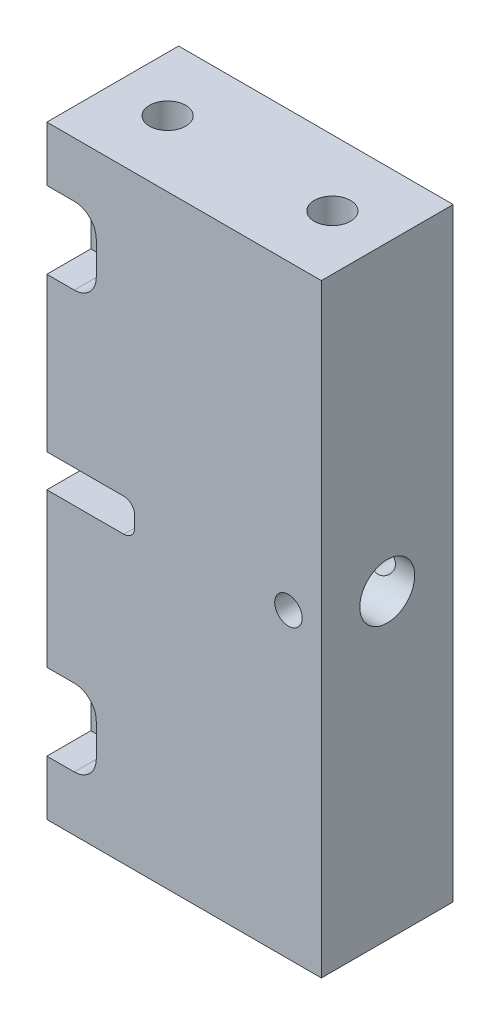
SolidWorks part; units mm, degrees
material "6061铝"
ref_plane "前视基准面" through (0, 0, 0) normal (0, 0, 1) x (1, 0, 0)
ref_plane "上视基准面" through (0, 0, 0) normal (0, 1, 0) x (1, 0, 0)
ref_plane "右视基准面" through (0, 0, 0) normal (1, 0, 0) x (0, 0, -1)
sketch "草图1" plane through (0, 0, 0) normal (1, 0, 0) x (0, 0, -1)
  line L1 (-6, 27.5) -> (6, 27.5)
  line L2 (-6, 27.5) -> (-6, -27.5)
  line L3 (-6, -27.5) -> (6, -27.5)
  line L4 (6, 27.5) -> (6, -27.5)
  line L5 (-6, 27.5) -> (6, -27.5) construction
  line L6 (-6, -27.5) -> (6, 27.5) construction
  point P0 (0, 0)
  dimension "D1" = 12
  dimension "D2" = 55
extrude "凸台-拉伸1" add sketch "草图1" along normal blind 25
sketch "草图2" plane through (25, 0, 0) normal (1, 0, 0) x (0, 0, -1)
  circle A0 centre (0, 0) radius 1.1
  dimension "D1" = 2.2
extrude "切除-拉伸1" cut sketch "草图2" against normal blind 25
sketch "草图3" plane through (25, 0, 0) normal (1, 0, 0) x (0, 0, -1)
  circle A0 centre (0, 0) radius 2.5
  dimension "D1" = 5
extrude "切除-拉伸2" cut sketch "草图3" against normal blind 8
chamfer "倒角1" [suppressed] distance 1 angle 45
sketch "草图4" plane through (0, 0, 6) normal (0, 0, 1) x (1, 0, 0)
  line L0 (0, 27.5) -> (0, -27.5) construction
  line L1 (-8, 1.5) -> (8, 1.5)
  line L2 (-8, 1.5) -> (-8, -1.5)
  line L3 (-8, -1.5) -> (8, -1.5)
  line L4 (8, 1.5) -> (8, -1.5)
  line L5 (-8, 1.5) -> (8, -1.5) construction
  line L6 (-8, -1.5) -> (8, 1.5) construction
  point P0 (0, 0)
  dimension "D1" = 8
  dimension "D2" = 3
extrude "切除-拉伸3" cut sketch "草图4" against normal blind 6
hole_wizard "M4 螺纹孔1" positions "草图6" profile "草图7" tap size "M4" standard "GB"
sketch "草图6" plane through (0, 27.5, 0) normal (0, 1, 0) x (1, 0, 0)
  line L3 (12.5, 6) -> (12.5, -10.1356) construction
  line L4 (25, 6) -> (0, 6) construction
  point P0 (5, 0)
  point P14 (20, 0)
  dimension "D1" = 15
sketch "草图7" plane through (5, 27.5, 0) normal (1, 0, 0) x (0, 0, 1)
  line L0 (0, 0) -> (0, 11.0914)
  line L1 (0, 11.0914) -> (1.65, 10.1)
  line L2 (1.65, 10.1) -> (1.65, 0)
  line L5 (1.65, 0) -> (0, 0)
  line L10 (0, 11.0914) -> (-1.65, 10.1) construction
  line L11 (0, -6.35) -> (0, 107.95) construction
  dimension "螺纹孔钻头直径" = 3.3
  dimension "螺纹孔钻头深度" = 10.1
  dimension "导头角度" = 118
cosmetic thread "孔螺蚊线1" parameters "D1"=8, "D2"=4
cosmetic thread "孔螺蚊线2" parameters "D1"=8, "D2"=4
mirror "镜向1" about plane through (0, 0, 0) normal (0, 1, 0) of "M4 螺纹孔1"
fillet "圆角1" radius 1 2 edges at (8, -1.5, 3) (8, 1.5, 3)
sketch "草图9" plane through (0, 0, 6) normal (0, 0, 1) x (1, 0, 0)
  line L1 (0, 27.5) -> (0, 1.5) construction
  line L2 (-4.5, 22.5) -> (2.5, 22.5)
  line L3 (-4.5, 22.5) -> (-4.5, 15.5)
  line L4 (-4.5, 15.5) -> (2.5, 15.5)
  line L5 (4.5, 20.5) -> (4.5, 17.5)
  line L6 (-4.5, 22.5) -> (4.5, 15.5) construction
  line L7 (0, 0) -> (40.0429, 0) construction
  line L8 (-4.5, 15.5) -> (4.5, 22.5) construction
  arc A0 (4.5, 17.5) -> (2.5, 15.5) centre (2.5, 17.5) cw
  arc A1 (4.5, 20.5) -> (2.5, 22.5) centre (2.5, 20.5) ccw
  point P0 (0, 19)
  dimension "D1" = 19
  dimension "D2" = 2
  dimension "D3" = 4.5
  dimension "D4" = 7
extrude "切除-拉伸4" cut sketch "草图9" against normal blind 4
mirror "镜向2" about plane through (0, 0, 0) normal (0, 1, 0) of "切除-拉伸4"
hole_wizard "M3 螺纹孔1" positions "草图10" profile "草图11" tap size "M3" standard "GB" end condition through all
sketch "草图10" plane through (0, 0, 6) normal (0, 0, 1) x (1, 0, 0)
  line L0 (25, 27.5) -> (25, -27.5) construction
  point P0 (22, 0)
  dimension "D1" = 3
sketch "草图11" plane through (22, 0, 6) normal (1, 0, 0) x (0, -1, 0)
  line L0 (0, 0) -> (0, 12)
  line L1 (0, 12) -> (1.25, 12)
  line L2 (1.25, 12) -> (1.25, 0)
  line L5 (1.25, 0) -> (0, 0)
  line L11 (0, -6.35) -> (0, 107.95) construction
  dimension "通孔螺纹孔钻头直径" = 2.5
  dimension "通孔螺纹孔钻头深度" = 12
cosmetic thread "孔螺蚊线3" parameters "D2"=3
chamfer "倒角2" [suppressed] distance 0.5 angle 45
fillet "圆角2" radius 1 1 edges at (17, 0, -1.1)
